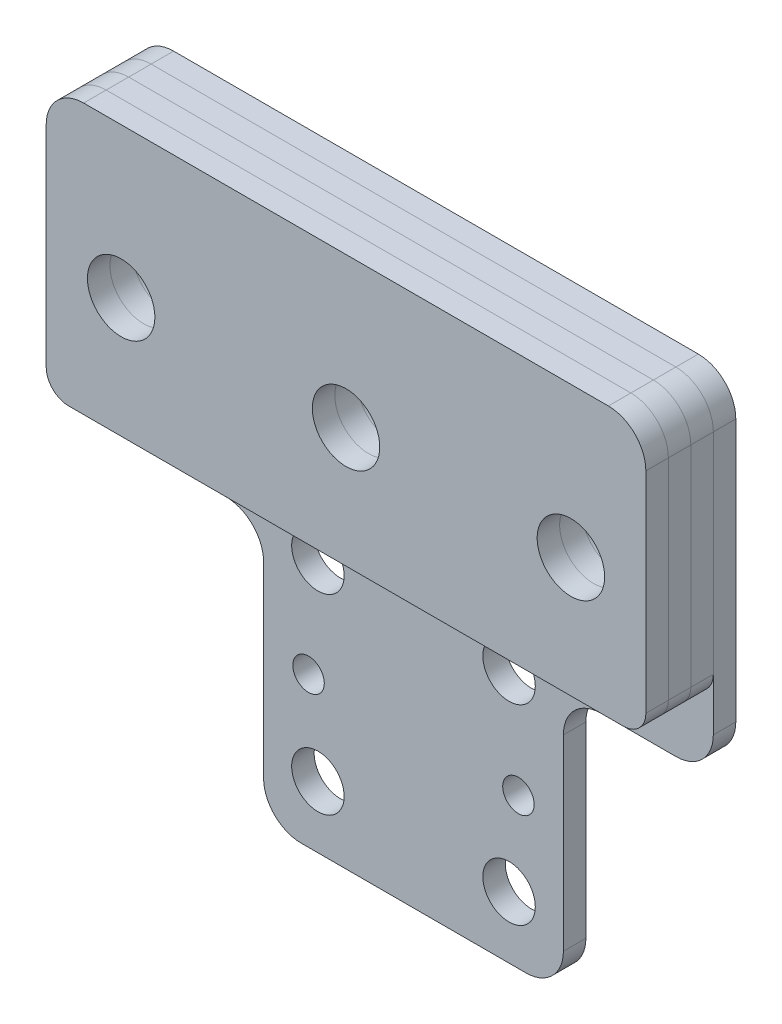
SolidWorks part; units mm, degrees
ref_plane "前视基准面" through (0, 0, 0) normal (0, 0, 1) x (1, 0, 0)
ref_plane "上视基准面" through (0, 0, 0) normal (0, 1, 0) x (1, 0, 0)
ref_plane "右视基准面" through (0, 0, 0) normal (1, 0, 0) x (0, 0, -1)
sketch "草图1" plane through (0, 0, 0) normal (0, 0, 1) x (1, 0, 0)
  line L1 (-40, 40) -> (40, 40)
  line L2 (-40, 40) -> (-40, -40)
  line L3 (-40, -40) -> (40, -40)
  line L4 (40, 40) -> (40, -40)
  line L5 (-40, 40) -> (40, -40) construction
  line L6 (-40, -40) -> (40, 40) construction
  point P0 (0, 0)
  dimension "D1" = 80
  dimension "D2" = 80
extrude "凸台-拉伸1" add sketch "草图1" along normal blind 3
sketch "草图5" plane through (0, 0, 3) normal (0, 0, 1) x (1, 0, 0)
  line L0 (0, -40) -> (0, -5.7146) construction
  line L1 (40, -40) -> (20, -40)
  line L2 (40, -40) -> (40, -5)
  line L3 (40, -5) -> (20, -5)
  line L4 (20, -40) -> (20, -5)
  line L5 (-40, -40) -> (40, -40) construction
  line L6 (-20, -40) -> (-20, -5)
  line L7 (-40, -5) -> (-20, -5)
  line L8 (-40, -40) -> (-40, -5)
  line L9 (-40, -40) -> (-20, -40)
  dimension "D1" = 20
  dimension "D2" = 35
extrude "切除-拉伸3" cut sketch "草图5" against normal blind 3
fillet "圆角1" radius 5 6 edges at (40, 40, 1.5) (-40, 40, 1.5) (20, -40, 1.5) (-20, -40, 1.5) (40, -5, 1.5) (-40, -5, 1.5)
sketch "草图2" plane through (0, 0, 3) normal (0, 0, 1) x (1, 0, 0)
  line L0 (0, 40) -> (0, 20) construction
  line L1 (35, 40) -> (-35, 40) construction
  line L2 (0, 20) -> (-30, 20) construction
  line L3 (0, 20) -> (30, 20) construction
  circle A0 centre (-30, 20) radius 4.5
  circle A1 centre (0, 20) radius 4.5
  circle A2 centre (30, 20) radius 4.5
  dimension "D3" = 9
  dimension "D1" = 60
  dimension "D2" = 20
extrude "切除-拉伸1" cut sketch "草图2" against normal blind 3
sketch "草图3" plane through (0, 0, 3) normal (0, 0, 1) x (1, 0, 0)
  line L0 (0, -40) -> (0, -19) construction
  line L1 (-15, -40) -> (15, -40) construction
  line L2 (35, 40) -> (-35, 40) construction
  line L3 (-12.75, -6.25) -> (12.75, -6.25) construction
  line L4 (-12.75, -6.25) -> (-12.75, -31.75) construction
  line L5 (-12.75, -31.75) -> (12.75, -31.75) construction
  line L6 (12.75, -6.25) -> (12.75, -31.75) construction
  line L7 (-12.75, -6.25) -> (12.75, -31.75) construction
  line L8 (-12.75, -31.75) -> (12.75, -6.25) construction
  circle A0 centre (12.75, -6.25) radius 3.5
  circle A1 centre (12.75, -31.75) radius 3.5
  circle A2 centre (-12.75, -31.75) radius 3.5
  circle A3 centre (-12.75, -6.25) radius 3.5
  dimension "D3" = 7
  dimension "D1" = 25.5
  dimension "D2" = 25.5
  dimension "D4" = 59
extrude "切除-拉伸2" cut sketch "草图3" against normal blind 3
sketch "草图4" plane through (0, 0, 3) normal (0, 0, 1) x (1, 0, 0)
  line L0 (-40, 4) -> (40, 4)
  line L1 (-40, 35) -> (-40, 0) construction
  line L2 (40, 0) -> (40, 35) construction
  line L3 (35, 40) -> (-35, 40) construction
  line L8 (-15, -40) -> (15, -40)
  line L9 (40, 0) -> (40, 35)
  line L10 (35, 40) -> (-35, 40)
  line L11 (-40, 35) -> (-40, 0)
  line L13 (40, 4) -> (40, 35)
  line L14 (35, 40) -> (-35, 40)
  line L15 (-40, 35) -> (-40, 4)
  line L20 (-35, -5) -> (-20, -5)
  line L22 (-20, -5) -> (-20, -35)
  line L24 (20, -35) -> (20, -5)
  line L26 (20, -5) -> (35, -5)
  circle A0 centre (30, 20) radius 4.5 construction
  circle A1 centre (-30, 20) radius 4.5 construction
  circle A2 centre (0, 20) radius 4.5 construction
  circle A3 centre (30, 20) radius 4.5
  circle A4 centre (-30, 20) radius 4.5
  circle A5 centre (0, 20) radius 4.5
  arc A10 (15, -40) -> (20, -35) centre (15, -35) ccw
  arc A11 (40, 35) -> (35, 40) centre (35, 35) ccw
  arc A12 (-35, 40) -> (-40, 35) centre (-35, 35) ccw
  arc A15 (40, 35) -> (35, 40) centre (35, 35) ccw
  arc A16 (-35, 40) -> (-40, 35) centre (-35, 35) ccw
  arc A18 (-20, -35) -> (-15, -40) centre (-15, -35) ccw
  arc A22 (35, -5) -> (40, 0) centre (35, 0) ccw
  arc A24 (-40, 0) -> (-35, -5) centre (-35, 0) ccw
  dimension "D1" = 36
  dimension "D2" = 0
extrude "凸台-拉伸2" add sketch "草图4" along normal blind 3 separate body
fillet "圆角2" radius 3 2 edges at (-40, 4, 4.5) (40, 4, 4.5)
pattern_linear "阵列(线性)1" count 3 spacing 3 along (0, 0, 1) of bodies 105
sketch "草图6" plane through (0, 0, 0) normal (0, 0, -1) x (-1, 0, 0)
  line L0 (0, -40) -> (0, -16.7045) construction
  line L1 (15, -40) -> (-15, -40) construction
  line L2 (-20, -5) -> (-20, -35) construction
  circle A0 centre (-14, -20) radius 2.1
  circle A1 centre (14, -20) radius 2.1
  dimension "D1" = 4.2
  dimension "D2" = 20
  dimension "D3" = 6
extrude "切除-拉伸4" cut sketch "草图6" against normal blind 3
fillet "圆角3" radius 5 2 edges at (-20, -5, 1.5) (20, -5, 1.5)
